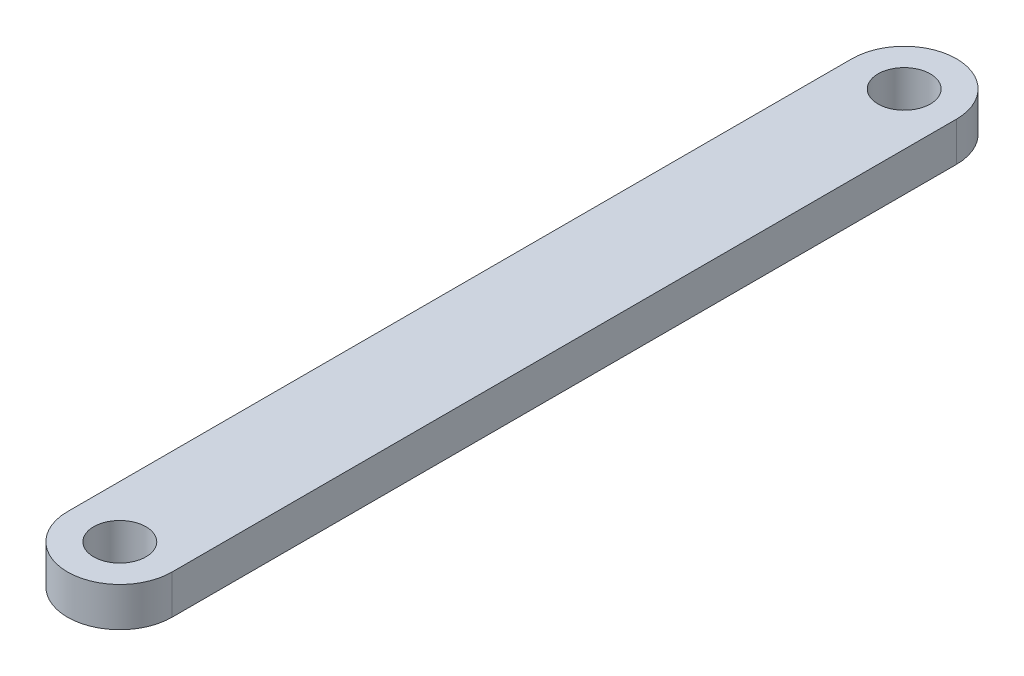
SolidWorks part; units mm, degrees
ref_plane "Front" through (0, 0, 0) normal (0, 0, 1) x (1, 0, 0)
ref_plane "Top" through (0, 0, 0) normal (0, 1, 0) x (1, 0, 0)
ref_plane "Right" through (0, 0, 0) normal (1, 0, 0) x (0, 0, -1)
sketch "Sketch1" plane through (0, 0, 0) normal (0, 1, 0) x (1, 0, 0)
  line L0 (0, 0) -> (0, 300) construction
  line L1 (-20, 0) -> (-20, 300)
  line L2 (20, 0) -> (20, 300)
  arc A0 (-20, 0) -> (20, 0) centre (0, 0) ccw
  arc A1 (20, 300) -> (-20, 300) centre (0, 300) ccw
  circle A2 centre (0, 300) radius 10
  circle A3 centre (0, 0) radius 10
  point P3 (0, 150)
  dimension "D2" = 20
  dimension "D3" = 20
  dimension "D4" = 20
  dimension "D1" = 300
extrude "Boss-Extrude1" add sketch "Sketch1" along normal blind 15
